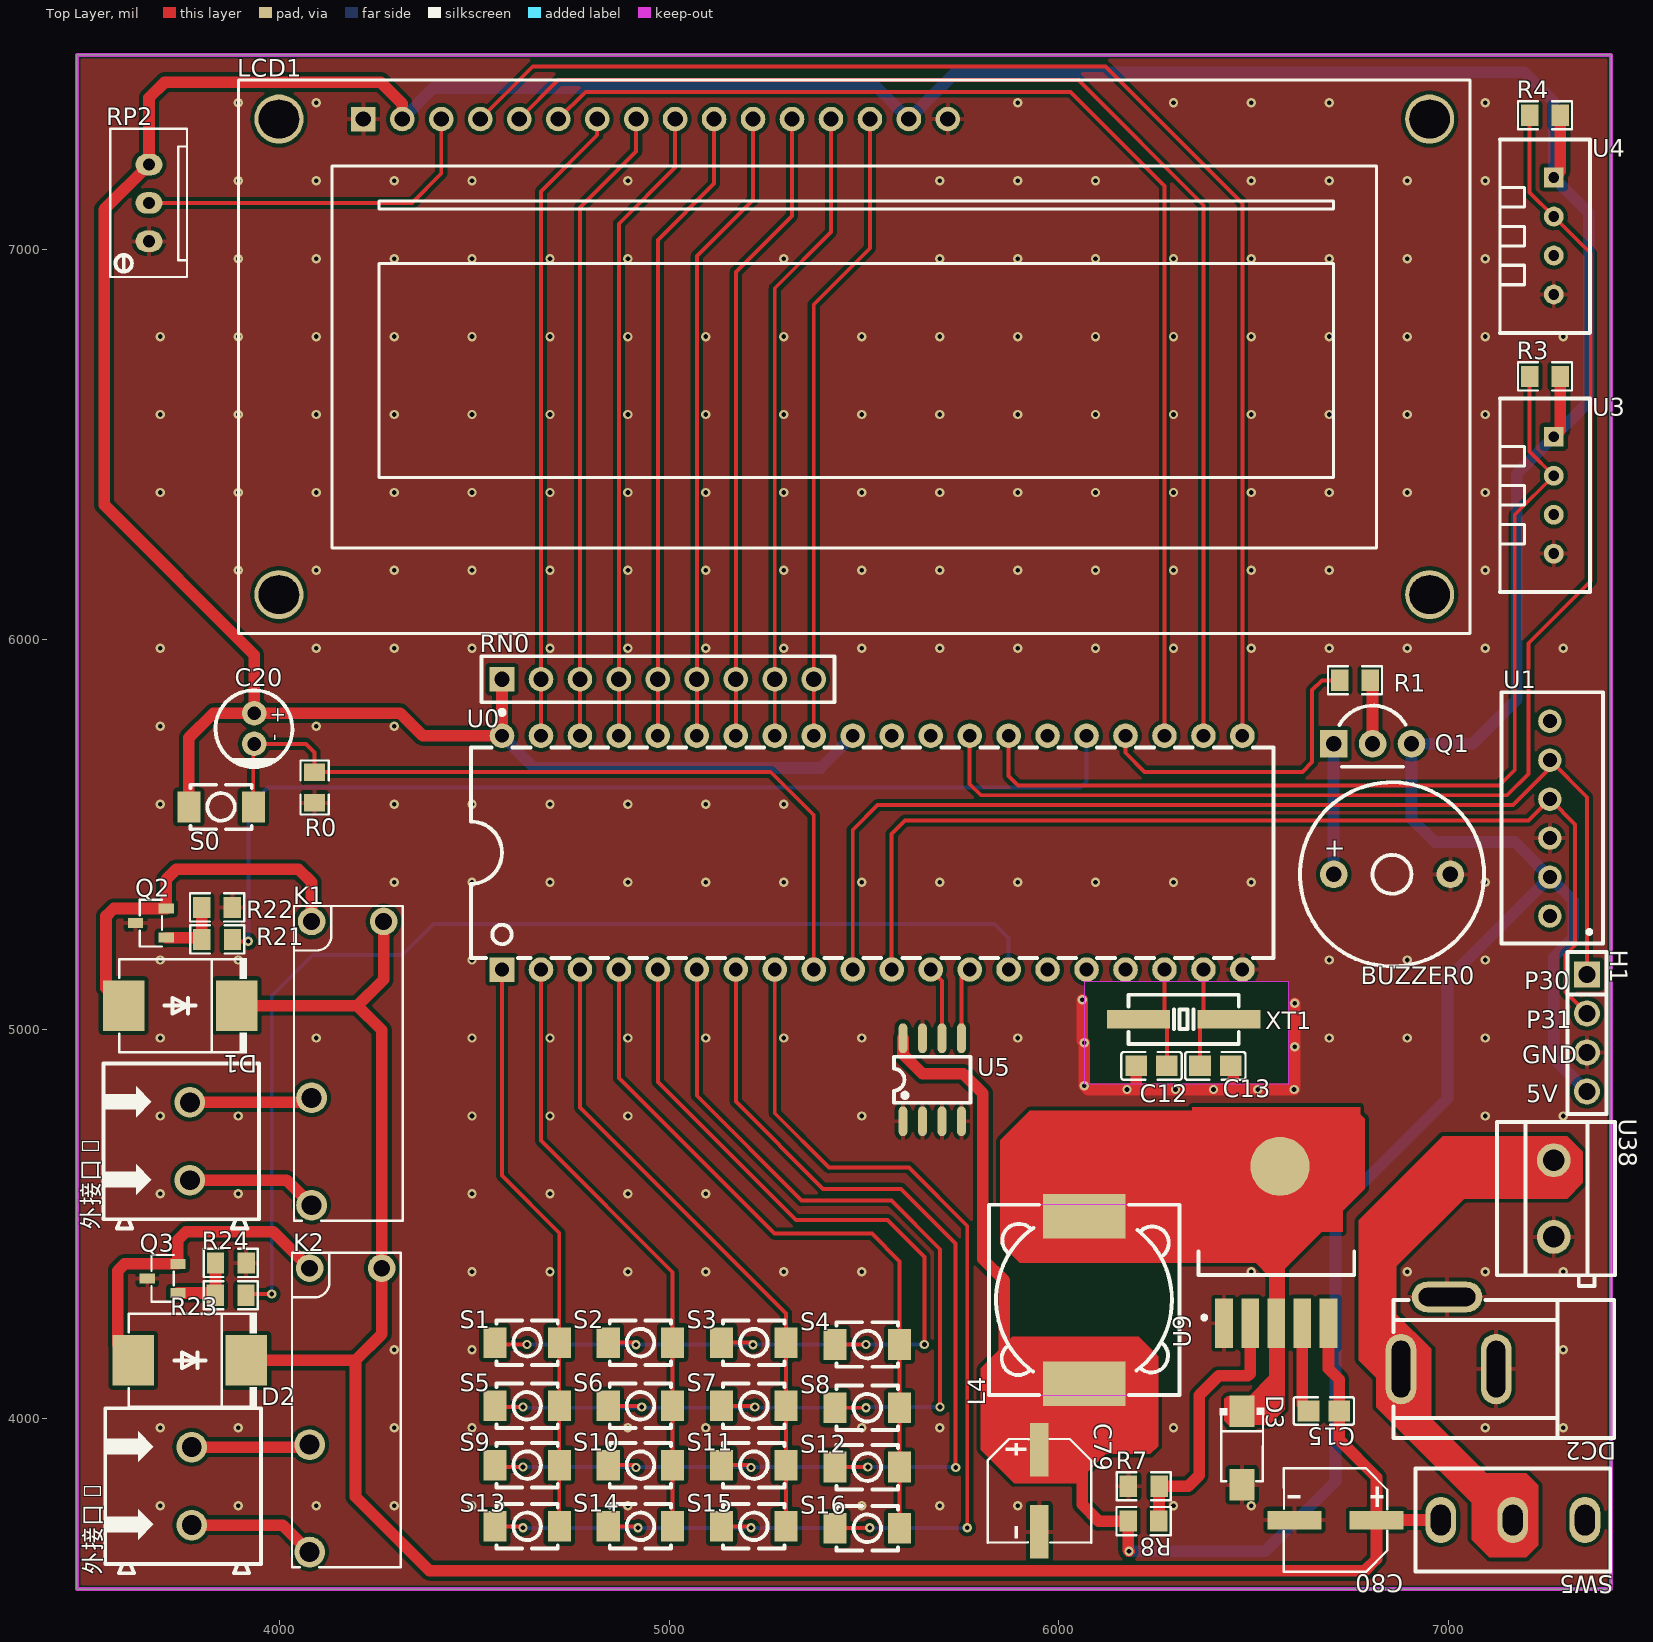
[diagram p0: Top Layer view]
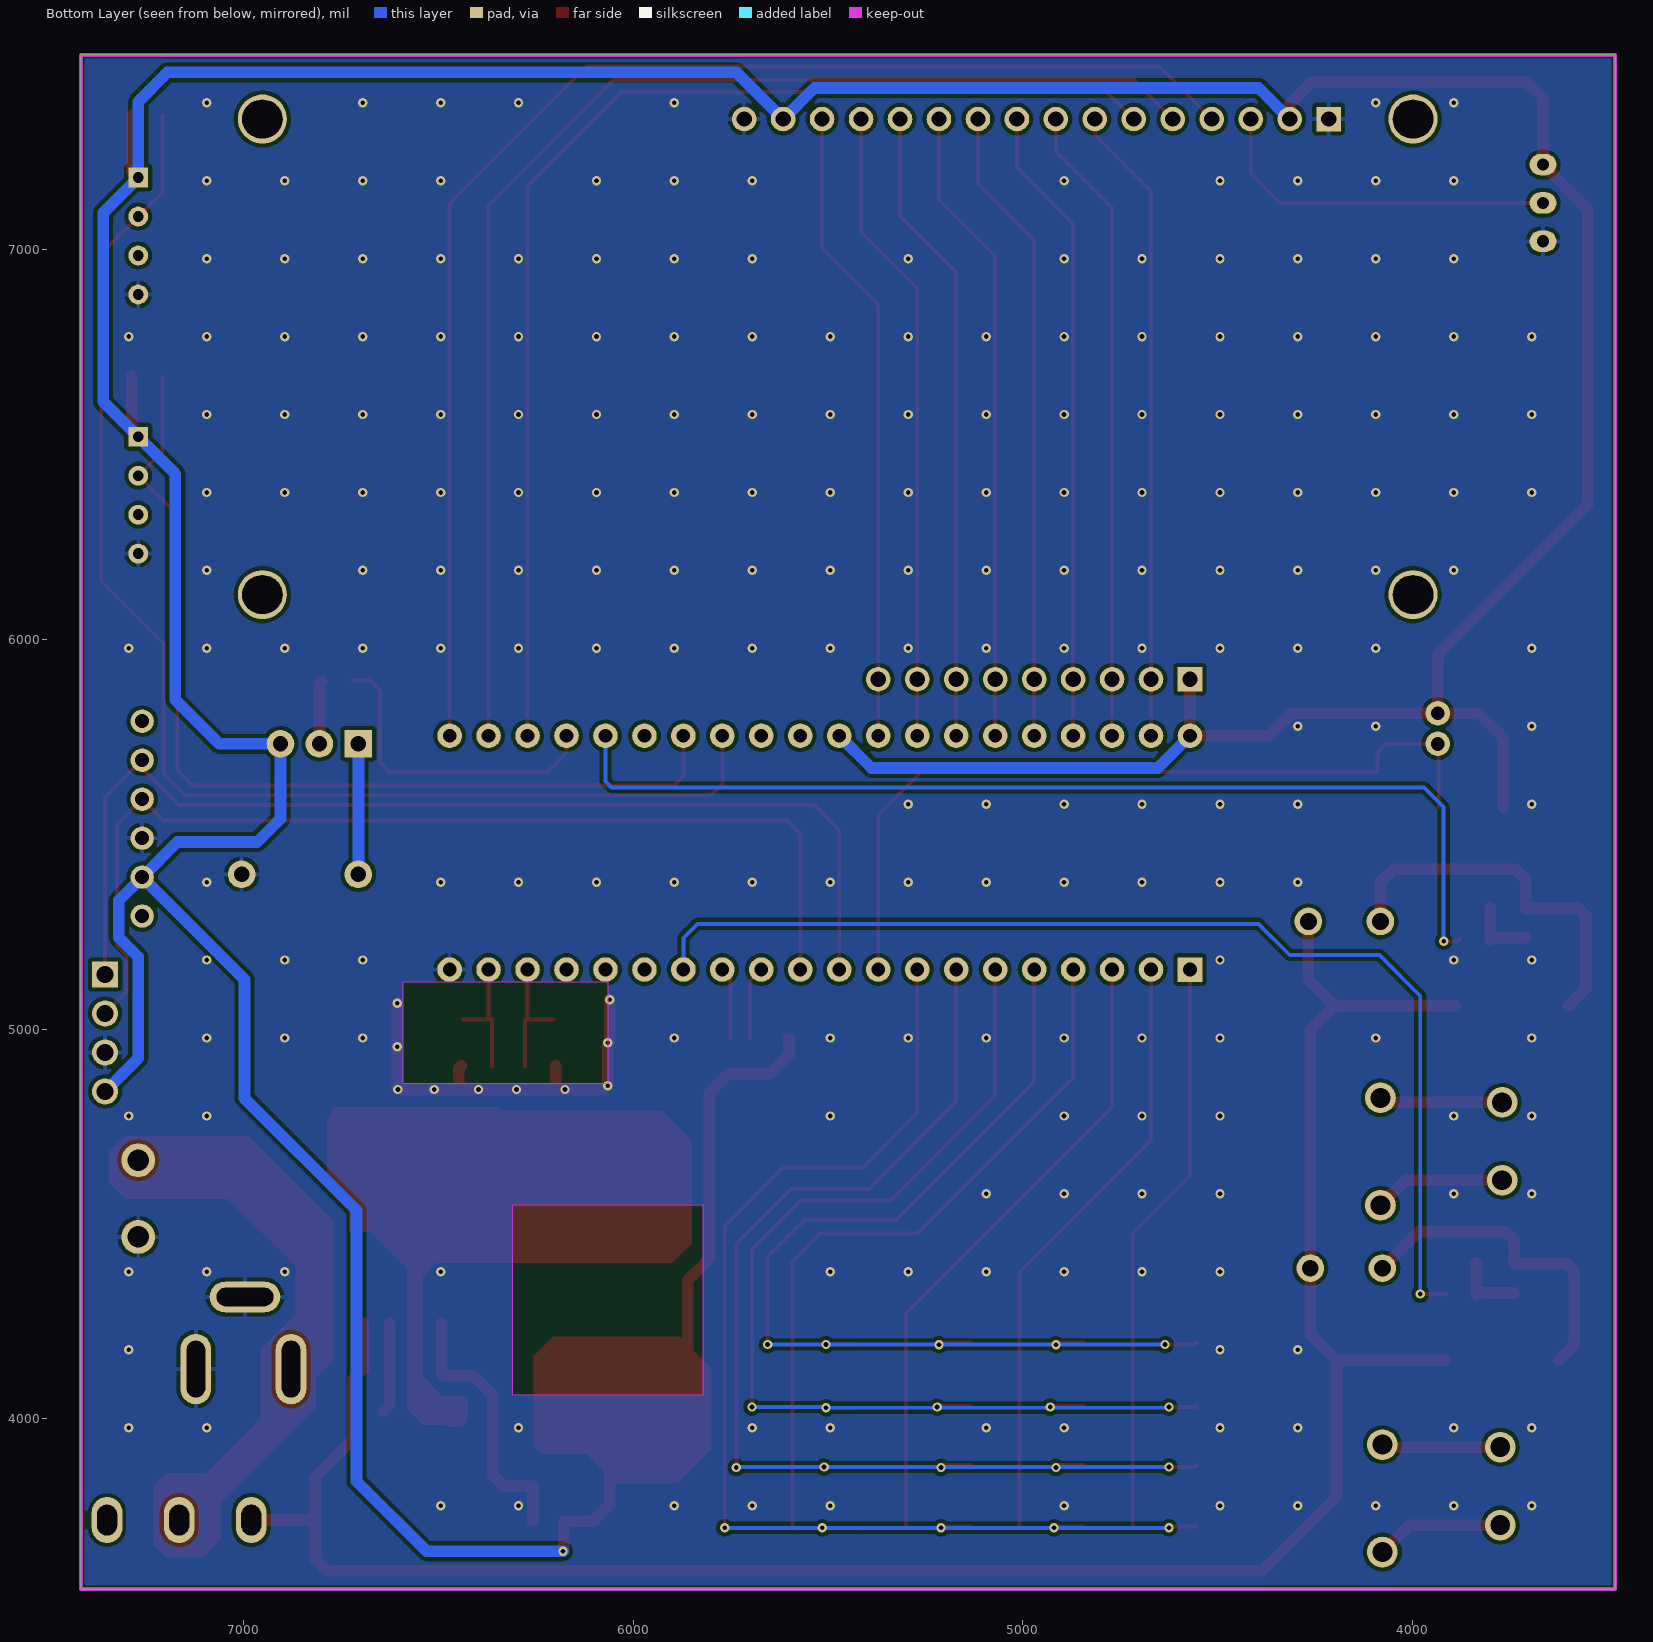
[diagram p1: Bottom Layer view, seen from below]
# Altium PCB MISC52141.pcbdoc
Units mil, origin at the board's own origin, x right, y up, seen from the top; angles counter-clockwise.
Board outline 3937.01 x 3937.01 mil, 2 copper layers (Top Layer, Bottom Layer), stack 62.206 mil thick; 59 components, 49 nets, 211 pads, 246 vias.

## Layer stack, top to bottom
Top Solder Mask Layer: solder mask 0.394, Dk 3.3
Top Layer: signal copper 1.379
Dielectric1: surface 59.449, FR4, Dk 4.5
Bottom Layer: signal copper 1.378
Bottom Solder Mask Layer: solder mask 0.394, Dk 3.3

## Board outline
3480,7500 3480,3562.99 7417.01,3562.99 7417.01,7500

## Design rules (kind name [scope] priority, off if disabled: settings)
BoardOutlineClearance copperThickness2oz_1 [All] p2 off: genericclearance=7.99 ignorepadtopadclearanceinfootprint=FALSE except(0: Arc-SplitContinuation Track-SplitContinuation SMDPad-SplitContinuation THPad-SplitContinuation Via-SplitContinuation Fill-SplitContinuation Region-SplitContinuation Poly-SplitContinuation Text-SplitContinuation Hole-SplitContinuation; 5.98: Arc-CutoutEdge SMDPad-CutoutEdge THPad-CutoutEdge Via-CutoutEdge Fill-CutoutEdge Region-CutoutEdge Text-CutoutEdge; 6.93: Hole-OutlineEdge Hole-CutoutEdge; 10: Poly-OutlineEdge Poly-CutoutEdge; 11.81: Arc-OutlineEdge Track-OutlineEdge SMDPad-OutlineEdge THPad-OutlineEdge Via-OutlineEdge Fill-OutlineEdge Region-OutlineEdge Text-OutlineEdge Track-CutoutEdge)
BoardOutlineClearance copperThickness1oz_1 [All] p4: genericclearance=4.02 ignorepadtopadclearanceinfootprint=FALSE except(0: Arc-SplitContinuation Track-SplitContinuation SMDPad-SplitContinuation THPad-SplitContinuation Via-SplitContinuation Fill-SplitContinuation Region-SplitContinuation Poly-SplitContinuation Text-SplitContinuation Hole-SplitContinuation; 6: SMDPad-CutoutEdge THPad-CutoutEdge Via-CutoutEdge Fill-CutoutEdge Region-CutoutEdge Text-CutoutEdge; 6.93: Hole-OutlineEdge Hole-CutoutEdge; 10: Poly-OutlineEdge Poly-CutoutEdge; 11.8: Arc-OutlineEdge Track-OutlineEdge SMDPad-OutlineEdge THPad-OutlineEdge Via-OutlineEdge Fill-OutlineEdge Region-OutlineEdge Text-OutlineEdge; 11.81: Arc-CutoutEdge Track-CutoutEdge)
Clearance copperThickness2oz [All] p1 off: gap=7.99 ignorepadtopadclearanceinfootprint=FALSE except(5.98: SMDPad-Track SMDPad-SMDPad THPad-Track SMDPad-THPad THPad-THPad Track-Via SMDPad-Via THPad-Via Via-Via Fill-Track Region-Track Fill-SMDPad Region-SMDPad Fill-THPad Region-THPad Fill-Via Region-Via Fill-Fill Fill-Region Region-Region Arc-Track Arc-SMDPad Arc-THPad Arc-Via Fill-Arc Region-Arc Arc-Arc Text-Track SMDPad-Text Text-THPad Text-Via Fill-Text Region-Text Arc-Text Text-Text; 6.93: Hole-Track Hole-SMDPad Hole-THPad Hole-Via Fill-Hole Region-Hole Hole-Arc Hole-Text; 10: Poly-Track Poly-SMDPad Poly-THPad Poly-Via Poly-Fill Poly-Region Poly-Poly Poly-Arc Poly-Text Poly-Hole)
Clearance copperThickness1oz [All] p3: gap=4.02 ignorepadtopadclearanceinfootprint=FALSE except(5.98: SMDPad-Track SMDPad-SMDPad THPad-Track SMDPad-THPad THPad-THPad Track-Via SMDPad-Via THPad-Via Via-Via Fill-Track Region-Track Fill-SMDPad Region-SMDPad Fill-THPad Region-THPad Fill-Via Region-Via Fill-Fill Fill-Region Region-Region; 6: Arc-Track Arc-SMDPad Arc-THPad Arc-Via Fill-Arc Region-Arc Arc-Arc Text-Track SMDPad-Text Text-THPad Text-Via Fill-Text Region-Text Arc-Text Text-Text; 6.93: Hole-Track Hole-SMDPad Hole-THPad Hole-Via Fill-Hole Region-Hole Hole-Arc Hole-Text; 10: Poly-Track Poly-SMDPad Poly-THPad Poly-Via Poly-Fill Poly-Region Poly-Poly Poly-Arc Poly-Text Poly-Hole)
DiffPairsRouting differentialPair [All] p1: maxlimit=6 minlimit=6 mostfreqgap=6 toplayer_minwidth=5 toplayer_prefwidth=10 toplayer_maxwidth=100 toplayer_mingap=6 toplayer_prefgap=6 toplayer_maxgap=6 bottomlayer_minwidth=5 bottomlayer_prefwidth=10 bottomlayer_maxwidth=100 bottomlayer_mingap=6 bottomlayer_prefgap=6 bottomlayer_maxgap=6 maxuncoupledlength=10
HoleToHoleClearance otherClearance [All] p1: gap=11.81 allowstackedmicrovias=TRUE
Length netLength [All] p1: minlimit=0 maxlimit=0
MatchedLengths netLengthTolerance [All] p1: tolerance=1000
PasteMaskExpansion pasteMaskExpansion [All] p1: expansion=0
PlaneConnect innerPlane [All] p1: planeconnectstyle=Relief reliefexpansion=20 reliefentries=4 reliefconductorwidth=10 reliefairgap=10
PolygonConnect copperRegion [(InNet('GND'))] p1: connectstyle=Relief reliefconductorwidth=10 reliefentries=4 polygonreliefangle="90 Angle" airgapwidth=10 via.connectstyle=Relief via.reliefconductorwidth=10 via.reliefentries=4 via.polygonreliefangle="90 Angle" via.airgapwidth=10
RoutingVias viaSize [All] p1: holewidth=12.01 width=24.02 viastyle="Through Hole" minholewidth=11.81 minwidth=19.68 maxholewidth=248.03 maxwidth=393.7
SolderMaskExpansion solderMaskExpansion [IsVia] p1: expansion=-1000 istentingtop=TRUE
SolderMaskExpansion solderMaskExpansion [All] p2: expansion=2 istentingtop=FALSE
Width copperThickness2oz_2 [All] p1 off: maxlimit=100 minlimit=8 preferedwidth=10
Width copperThickness1oz_2 [All] p2: maxlimit=100 minlimit=5 preferedwidth=10

## Components (designator, comment, footprint, x,y, rotation, side; value= is the part's Value field where it differs from the comment)
BUZZER0 "2.4kHz" BUZ-TH_BD12.0-P7.60-D0.6-FD 6855,5397.11 r0 top
C12 "30pf" C0805 6237.82,4905.52 r180 top
C13 "30pf" C0805 6401.58,4905.52 r0 top
C15 "100nF" C0805 6680,4020 r180 top
C20 "CAP-E" CAP-TH_BD5.0-P2.00-D0.5-FD-A 3935.01,5771.26 r270 top
C79 "100uF" CAP-SMD_BD6.3-L6.6-W6.6-LS7.4-FD 5950,3815 r270 top
C80 "100uF" CAP-SMD_BD6.3-L6.6-W6.6-LS7.4-FD 6710,3740 r180 top
D1 "" SMC_L6.9-W5.9-LS7.9-RD 3745,5060 r180 top
D2 "" SMC_L6.9-W5.9-LS7.9-RD 3770,4150 r180 top
D3 "SS510" SMA_L4.3-W2.6-LS5.0-RD 6470,3925 r270 top
DC2 "DC005" DC-IN-TH_DC005 7000,4220 r180 top
H1 "" HDR-TH_4P-P2.54-V-F 7355,4990 r270 top
K1 "" RELAY-TH_G5NB-1A-E-DCXX 4174.81,4912.09 r270 top
K2 "" RELAY-TH_G5NB-1A-E-DCXX 4169.81,4022.09 r270 top
L4 "47uH" IND-SMD_L12.3-W12.3 6065,4305 r90 top
LCD1 "LCD 1602" LCD1602 5475,6725 r0 top
Q1 "SS8550DTA" TO-92-3_L4.8-W3.7-P2.54-L 6805,5732.11 r0 top
Q2 "S8050(0.5A)" SOT-23-3_L2.9-W1.3-P1.90-LS2.4-BR 3669.81,5272.09 r0 top
Q3 "S8050(0.5A)" SOT-23-3_L2.9-W1.3-P1.90-LS2.4-BR 3700,4360 r0 top
R0 "10K" R0805 4090,5620 r90 top
R1 "5.1K" R0805 6760,5895 r0 top
R3 "10K" R0805 7247.35,6675 r0 top
R4 "10K" R0805 7247.35,7345 r0 top
R7 "3.3K" R0805 6217.85,3826.84 r0 top
R8 "10K" R0805 6217.38,3737.37 r180 top
R21 "4.7K" R0805 3840,5230 r0 top
R22 "4.7K" R0805 3839.81,5312.09 r180 top
R23 "4.7K" R0805 3874.81,4317.09 r0 top
R24 "4.7K" R0805 3875,4400 r180 top
RN0 "10kΩ" RES-ARRAY-TH_9P-P2.54-D1.0 4971,5897.74 r0 top
RP2 "10K" RES-ADJ-TH_3296W-1-203 3665,7119.99 r270 top
S0 "SW2" SW-SMD_L3.9-W2.9-LS5.0 3850,5570 r180 top
S1 "SW2" SW-SMD_L3.9-W2.9-LS5.0 4635.31,4195.44 r0 top
S2 "SW2" SW-SMD_L3.9-W2.9-LS5.0 4926.31,4195.44 r0 top
S3 "SW2" SW-SMD_L3.9-W2.9-LS5.0 5217.31,4195.44 r0 top
S4 "SW2" SW-SMD_L3.9-W2.9-LS5.0 5508.31,4190.44 r0 top
S5 "SW2" SW-SMD_L3.9-W2.9-LS5.0 4635.31,4033.23 r0 top
S6 "SW2" SW-SMD_L3.9-W2.9-LS5.0 4926.31,4033.23 r0 top
S7 "SW2" SW-SMD_L3.9-W2.9-LS5.0 5217.32,4033.23 r0 top
S8 "SW2" SW-SMD_L3.9-W2.9-LS5.0 5508.32,4028.23 r0 top
S9 "SW2" SW-SMD_L3.9-W2.9-LS5.0 4635.31,3881.03 r0 top
S10 "SW2" SW-SMD_L3.9-W2.9-LS5.0 4926.31,3881.03 r0 top
S11 "SW2" SW-SMD_L3.9-W2.9-LS5.0 5217.32,3881.03 r0 top
S12 "SW2" SW-SMD_L3.9-W2.9-LS5.0 5508.32,3876.03 r0 top
S13 "SW2" SW-SMD_L3.9-W2.9-LS5.0 4635.31,3723.82 r0 top
S14 "SW2" SW-SMD_L3.9-W2.9-LS5.0 4926.31,3723.82 r0 top
S15 "SW2" SW-SMD_L3.9-W2.9-LS5.0 5217.32,3723.82 r0 top
S16 "SW2" SW-SMD_L3.9-W2.9-LS5.0 5508.32,3718.82 r0 top
SW5 "SS-12D10L5" SW-TH_SS-12D10L5 7165,3740 r180 top
U0 "STC89C52RC-40I-PDIP40" DIP-40_L52.0-W13.7-P2.54-LS15.2-BL 5521,5452.74 r0 top
U1 "HM-10" HM-10.288 7260,5290 r180 top
U3 "DHT11" SENSOR-TH_DHT11 7270,6370 r270 top
U4 "DHT11" SENSOR-TH_DHT11 7270,7035 r270 top
U5 "M24C64-RMN6TP" SOIC-8_L5.0-W4.0-P1.27-LS6.0-BL 5675,4870 r0 top
U9 "XL4015E1" TO-263-5_L10.2-W8.9-P1.70-TL 6557.88,4442.34 r90 top
U38 "KF301-5.0-2P" CONN-TH_P5.00_KF301-5.0-2P 7270,4565 r270 top
XT1 "XT" HC-49S_L7.2-W3.2 6320,5025 r180 top
外接口1 "" CONN-TH_2P-P5.00_WJ500V-5.08-2P 3769.81,4712.09 r90 top
外接口2 "" CONN-TH_2P-P5.00_WJ500V-5.08-2P 3774.81,3827.09 r90 top

## Footprints (in the part's own frame and the unit in brackets; to place one, negate y for a bottom-side part, rotate by r counter-clockwise, add the part's x,y. Pads: shape width x height; smd on the part's side, far side on the other; paste and mask are expansions set on the pad)
BUZ-TH_BD12.0-P7.60-D0.6-FD [mm]
  round 1.8 hole 1: 1(-3.8,0) 2(3.8,0)
  silkscreen extent -6,-6 6,6
C0805 [mm]
  rect 1.41x1.35 smd paste-100 mask+0.051: 1(-1,0) 2(1,0)
  silkscreen extent -1.96,-0.9 1.96,0.9
CAP-SMD_BD6.3-L6.6-W6.6-LS7.4-FD [mm]
  rect 3.5x1.2 smd: 1(-2.67,0) 2(2.67,0)
  silkscreen extent -3.38,-3.38 3.38,3.38
CAP-TH_BD5.0-P2.00-D0.5-FD-A [mm]
  round 1.6 hole 0.9 paste+0 mask+0.05: 1(-1,0) 2(1,0)
  silkscreen extent -2.49,-2.52 2.6,2.49
CONN-TH_2P-P5.00_WJ500V-5.08-2P [mm]
  round 2 hole 1.3: 1(-2.54,0) 2(2.54,0)
  silkscreen extent -5.68,-4.52 5.08,5.64
CONN-TH_P5.00_KF301-5.0-2P [mm]
  round 2.2 hole 1.4: 1(-2.5,0) 2(2.5,0)
  silkscreen extent -5,-3.7 5.71,4
DC-IN-TH_DC005 [mm]
  oval 2x4.6 hole 1.2 slot 3.7 at 90 deg: 1(3.1,2.35) 2(-3.1,2.35)
  oval 4.6x2 hole 1.2 slot 3.7 at 0 deg: 3(0.1,-2.35)
  silkscreen extent -10.8,-2.15 3.6,6.85
DIP-40_L52.0-W13.7-P2.54-LS15.2-BL [mil]
  rect 63x63 hole 35: 1(-950,-300)
  round 63 hole 35: 2(-850,-300) 3(-750,-300) 4(-650,-300) 5(-550,-300) 6(-450,-300) 7(-350,-300) 8(-250,-300) 9(-150,-300) 10(-50,-300) 11(50,-300) 12(150,-300) 13(250,-300) 14(350,-300) 15(450,-300) 16(550,-300) 17(650,-300) 18(750,-300) 19(850,-300) 20(950,-300) 21(950,300) 22(850,300) 23(750,300) 24(650,300) 25(550,300) 26(450,300) 27(350,300) 28(250,300) 29(150,300) 30(50,300) 31(-50,300) 32(-150,300) 33(-250,300) 34(-350,300) 35(-450,300) 36(-550,300) 37(-650,300) 38(-750,300) 39(-850,300) 40(-950,300)
  silkscreen extent -1030,-270 1030,270
HC-49S_L7.2-W3.2 [mm]
  rect 4.1x1.2 smd: 1(-2.95,0) 2(2.95,0)
  silkscreen extent -3.6,-1.6 3.6,1.6
HDR-TH_4P-P2.54-V-F [mm]
  rect 1.7x1.7 hole 1.1: 1(-3.81,0)
  round 1.7 hole 1.1: 2(-1.27,0) 3(1.27,0) 4(3.81,0)
  silkscreen extent -5.29,-1.27 5.29,1.27
HM-10.288 [mil]
  round 60 hole 36: 1(0,0) 2(0,-100) 3(0,-200) 4(0,-300) 5(0,-400) 6(0,-500)
  silkscreen extent -136,-574 124,71
IND-SMD_L12.3-W12.3 [mm]
  rect 2.9x5.4 smd: 1(-5.45,0) 2(5.45,0)
  silkscreen extent -6.2,-6.2 6.2,6.2
LCD1602 [mm]
  round 3.2 hole 2.5 slot 2.625 at 0 deg: 0(-37.5,-15.5) 0(-37.5,15.5) 0(37.5,-15.5) 0(37.5,15.5)
  rect 1.6x1.6 hole 1: 1(-32,15.5)
  round 1.6 hole 1: 2(-29.46,15.5) 3(-26.92,15.5) 4(-24.38,15.5) 5(-21.84,15.5) 6(-19.3,15.5) 7(-16.76,15.5) 8(-14.22,15.5) 9(-11.68,15.5) 10(-9.14,15.5) 11(-6.6,15.5) 12(-4.06,15.5) 13(-1.52,15.5) 14(1.02,15.5) 15(3.56,15.5) 16(6.1,15.5)
  silkscreen extent -40.13,-18.03 40.13,18.03
R0805 [mm]
  rect 1.133x1.377 smd paste-100 mask+0.051: 1(-1,0) 2(1,0)
  silkscreen extent -1.76,-0.92 1.76,0.92
RELAY-TH_G5NB-1A-E-DCXX [mm]
  round 1.8 hole 1.1: 1(-9.25,-2.35) 4(-9.25,2.35)
  round 2 hole 1.3: 2(2.25,-2.35) 3(9.25,-2.35)
  silkscreen extent -10.25,-3.5 10.25,3.6
RES-ADJ-TH_3296W-1-203 [mm]
  oval 1.4x1.75 hole 0.8: 1(-2.5,0) 2(0,0) 3(2.5,0)
  silkscreen extent -4.83,-2.53 4.83,2.48
RES-ARRAY-TH_9P-P2.54-D1.0 [mm]
  rect 1.6x1.6 hole 1: 1(-10.16,0)
  round 1.6 hole 1: 2(-7.62,0) 3(-5.08,0) 4(-2.54,0) 5(0,0) 6(2.54,0) 7(5.08,0) 8(7.62,0) 9(10.16,0)
  silkscreen extent -11.5,-2.31 11.5,1.5
SENSOR-TH_DHT11 [mil]
  rect 51x51 hole 28: 1(-150,0)
  round 51 hole 28: 2(-50,0) 3(50,0) 4(150,0)
  silkscreen extent -248,-138 248,93
SMA_L4.3-W2.6-LS5.0-RD [mm]
  rect 2.046x1.62 smd: 1(-2.404,-0.009) 2(2.404,0.009)
  silkscreen extent -2.61,-1.44 2.16,1.44
SMC_L6.9-W5.9-LS7.9-RD [mm]
  rect 2.7x3.3 smd: 1(-3.686,0) 2(3.686,0)
  silkscreen extent -4.36,-3.1 3.98,3.1
SOIC-8_L5.0-W4.0-P1.27-LS6.0-BL [mil]
  oval 22.38x76.78 smd: 1(-75,-106.5) 2(-25,-106.5) 3(25,-106.5) 4(75,-106.5) 5(75,106.5) 6(25,106.5) 7(-25,106.5) 8(-75,106.5)
  silkscreen extent -98,-59 98,59
SOT-23-3_L2.9-W1.3-P1.90-LS2.4-BR [mm]
  rect 1x0.65 smd: 1(1,-0.95) 2(1,0.95) 3(-1,0)
  silkscreen extent -0.73,-1.53 0.73,1.53
SW-SMD_L3.9-W2.9-LS5.0 [mm]
  rect 1.5x2 smd: 1(-2.1,0) 2(2.1,0)
  silkscreen extent -2,-1.45 2,1.45
SW-TH_SS-12D10L5 [mm]
  oval 2x3 hole 1.3 slot 2 at 90 deg: 1(-4.7,0) 2(0,0) 3(4.7,0)
  silkscreen extent -6.35,-3.35 6.35,3.35
TO-92-3_L4.8-W3.7-P2.54-L [mm]
  rect 1.8x1.8 hole 1: 1(-2.54,0)
  round 1.8 hole 1: 2(0,0) 3(2.54,0)
  silkscreen extent -2.17,-1.5 2.14,2.48
TO-263-5_L10.2-W8.9-P1.70-TL [mm]
  rect 3.2x1.15 smd: 1(-5.008,3.404) 2(-5.008,1.702) 3(-5.008,0) 4(-5.008,-1.702) 5(-5.008,-3.404)
  round 3.852 smd: 6(5.219,-0.241)
  Top Layer region: 0.944,3.683 7.548,3.683 7.548,5.461 9.072,5.461 9.072,-5.461 7.548,-5.461 7.548,-4.317 0.944,-4.317
  silkscreen extent -4.77,-5.08 -0.33,5.08

## Via types
v1: diameter 24.02, hole 12, Top Layer to Bottom Layer, 246 vias

## Nets (pads, with @x,y where several pads share a name; then routed paths per layer and width w, separated by ;. In a path a pad name is that pad's centre, name@x,y a point inside that pad or via, vN(x,y) a via of type N, cw(c..) or ccw(c..) an arc to the next point about the centre after c; other vN are vias at no path point)
12V: C15.1 C80.1 D1.1 D2.1 K1.4 K2.4 SW5.3 U9.5 | length 5679.8
  Top Layer w30: D1.1 4200,5060 ; D2.1 4195,4150 ; K1.4 4267.33,5127.33 4200,5060 ; U9.5 6691.88,4128.12 6719.37,4100.63 C15.1 6719.37,3945.63 6815.11,3849.89 C80.1 ; SW5.3 C80.1 ; 4195,4150 4262.33,4217.33 K2.4 4262.33,4997.67 4200,5060 ; 4195,4150 4195,3800 4385,3610 6785,3610 6815.11,3640.11 C80.1
$1N45: C20.2 R0.2 S0.1 U0.9 | length 2100.5
  Top Layer w10: S0.1 3932.68,5729.57 C20.2 4068.11,5731.89 4090,5710 R0.2 5260.63,5659.37 5371,5549 U0.9
$1N63: LCD1.3 RP2.2 | length 921.4
  Top Layer w10: RP2.2 4339.99,7119.99 4415.16,7195.16 LCD1.3
$1N105: Q1.2 R1.2 | length 162.3
  Top Layer w30: R1.2@6799.37,5892.11 6805,5886.48 Q1.2
$1N108: BUZZER0.1 Q1.1 | length 335.2
  Bottom Layer w30: Q1.1 6705,5397.51 BUZZER0.1
$1N929: K1.2 外接口1.2 | length 317.2
  Top Layer w30: 外接口1.2 4070.87,4812.09 K1.2
$1N930: K1.3 外接口1.1 | length 339.1
  Top Layer w30: 外接口1.1 4018.11,4612.09 K1.3
$1N931: D1.2 K1.1 Q2.2 | length 983.4
  Top Layer w30: D1.2 3555,5104.87 3555,5290 3574.49,5309.49 Q2.2 3709.18,5384.18 3735,5410 4048.79,5410 4082.29,5376.5 K1.1
$1N934: Q2.1 R21.1 R22.2 | length 175.3
  Top Layer w30: Q2.1 3795.94,5234.69 R21.1@3800.44,5230.19 ; R22.2 R21.1@3800.44,5230.19 ; R21.1 R21.1@3800.44,5230.19
$1N936: K2.2 外接口2.2 | length 305.1
  Top Layer w30: 外接口2.2 4070.87,3927.09 K2.2
$1N937: K2.3 外接口2.1 | length 331.1
  Top Layer w30: 外接口2.1 4008.11,3727.09 K2.3
$1N938: D2.2 K2.1 Q3.2 | length 855.8
  Top Layer w30: D2.2 3585,4189.87 3585,4380 3602.4,4397.4 Q3.2 3738.79,4397.98 3738.79,4458.79 3760,4480 3983.55,4480 K2.1
$1N941: Q3.1 R23.1 R24.2 | length 181.3
  Top Layer w30: Q3.1 3829.92,4322.6 R23.1 3835.63,4317.28 R24.2
$1N950: D3.1 L4.2 U9.3 U9.6 | length 1244.7
  Top Layer w30: L4.2 6450.45,4519.57 U9.6@6557.88,4627 ; D3.1 6544.65,4019.64 6560,4035 6560,4243.07 U9.3 U9.6@6557.88,4627 ; U9.6@6570.38,4639.5 U9.6@6557.88,4627
$1N952: C15.2 U9.4 | length 231.7
  Top Layer w30: U9.4 6624.88,4035.75 C15.2
$1N964: DC2.1 SW5.2 U38.1
+5V: C20.1 C79.1 H1.4 L4.1 LCD1.2 LCD1.15 Q1.3 R3.2 R4.2 R8.2 RN0.1 RP2.1 S0.2 U0.31 U0.40 U1.2 U3.1 U4.1 U5.8 | length 15136.3
  Top Layer w30: S0.2 3767.32,5747.32 3830.63,5810.63 C20.1 ; LCD1.2 4315.16,7374.84 4260,7430 3705,7430 3665,7390 RP2.1 3550,7103.41 3550,6345 3935,5960 C20.1 ; RN0.1 U0.40 4367.26,5752.74 4309.37,5810.63 C20.1 ; U5.8 5600,4935 5650,4885 5755,4885 5805,4835 5805,4410 5860,4355 5860,4120 ; C79.1 6004.89,3920.11 6060,3865 6060,3780 6102.63,3737.37 R8.2 6178.01,3661.99 v1(6180,3660) ; U3.1 7286.72,6536.72 R3.2 ; U4.1 7286.72,7201.72 R4.2
  Bottom Layer w30: LCD1.2 4394.92,7415 5535.4,7415 LCD1.15 5734.92,7455 7195,7455 7270,7380 U4.1 7360,7095 7360,6610 U3.1 7175,6425 7175,5845 7062.11,5732.11 Q1.3 6905,5540 6965,5480 7170,5480 U1.2 ; U0.40 4653.74,5670 5388.26,5670 U0.31 ; v1(6180,3660) 6530,3660 6710,3840 6710,4535 6997.5,4822.5 6997.5,5127.5 U1.2 ; H1.4 7270,4925 7270,5185 7320,5235 7320,5330 U1.2
FB: R7.2 R8.1 U9.2 | length 692.4
  Top Layer w30: R8.1 6256.75,3826.37 R7.2 6331.84,3826.84 6360,3855 6360,4060 6410,4110 6485,4110 6490.88,4115.88 U9.2
GND: BUZZER0.2 C12.2 C13.2 C79.2 C80.2 D3.2 DC2.2 DC2.3 H1.3 LCD1.1 LCD1.16 Q2.3 Q3.3 R0.1 R7.1 R22.1 R24.1 RP2.3 U0.20 U1.3 U3.4 U4.4 U5.1 U5.2 U5.3 U5.4 U5.7 U9.1 U38.2 | length 1110.9
  Top Layer w30: v1(6060,5075) 6060,4970 v1(6065,4965) v1(6065,4854.78) 6074.78,4845 v1(6175,4845) 6196.99,4845 ; C12.2 6198.45,4846.46 6196.99,4845 ; C13.2 6447.41,4899.06 6447.41,4845 ; v1(6605,5066.04) v1(6605,4955) 6605,4846.4 v1(6603.6,4845) v1(6510.71,4845) 6447.41,4845 ; 6196.99,4845 v1(6299.45,4845) v1(6396.88,4845) 6447.41,4845
  other v1: 3694.1,3777.09 3894.1,3777.09 4094.1,3777.09 4294.1,3777.09 4494.1,3777.09 4894.1,3777.09 5494.1,3777.09 5694.1,3777.09 5894.1,3777.09 6294.1,3777.09 6494.1,3777.09 3694.1,3977.09 3894.1,3977.09 4294.1,3977.09 4494.1,3977.09 4894.1,3977.09 5094.1,3977.09 5494.1,3977.09 5694.1,3977.09 6294.1,3977.09 7094.1,3977.09 7294.1,3977.09 4294.1,4177.09 4494.1,4177.09 7294.1,4177.09 4494.1,4377.09 4694.1,4377.09 4894.1,4377.09 5094.1,4377.09 5294.1,4377.09 5494.1,4377.09 6494.1,4377.09 6894.1,4377.09 7094.1,4377.09 7294.1,4377.09 3694.1,4577.09 3894.1,4577.09 4494.1,4577.09 4694.1,4577.09 4894.1,4577.09 5094.1,4577.09 3694.1,4777.09 3894.1,4777.09 4494.1,4777.09 4694.1,4777.09 4894.1,4777.09 5494.1,4777.09 7094.1,4777.09 7294.1,4777.09 3694.1,4977.09 4094.1,4977.09 4494.1,4977.09 4694.1,4977.09 4894.1,4977.09 5094.1,4977.09 5294.1,4977.09 5494.1,4977.09 5894.1,4977.09 6694.1,4977.09 6894.1,4977.09 7094.1,4977.09 3694.1,5177.09 3894.1,5177.09 4494.1,5177.09 6694.1,5177.09 6894.1,5177.09 7094.1,5177.09 4294.1,5377.09 4494.1,5377.09 4694.1,5377.09 4894.1,5377.09 5094.1,5377.09 5294.1,5377.09 5494.1,5377.09 5694.1,5377.09 5894.1,5377.09 6094.1,5377.09 6294.1,5377.09 6494.1,5377.09 7094.1,5377.09 3694.1,5577.09 4294.1,5577.09 4494.1,5577.09 4694.1,5577.09 4894.1,5577.09 5094.1,5577.09 5294.1,5577.09 3694.1,5777.09 4094.1,5777.09 4294.1,5777.09 3694.1,5977.09 4094.1,5977.09 4294.1,5977.09 4494.1,5977.09 4694.1,5977.09 4894.1,5977.09 5094.1,5977.09 5294.1,5977.09 5494.1,5977.09 5694.1,5977.09 5894.1,5977.09 6094.1,5977.09 6294.1,5977.09 6494.1,5977.09 6694.1,5977.09 6894.1,5977.09 7094.1,5977.09 7294.1,5977.09 3894.1,6177.09 4094.1,6177.09 4294.1,6177.09 4494.1,6177.09 4694.1,6177.09 4894.1,6177.09 5094.1,6177.09 5294.1,6177.09 5494.1,6177.09 5694.1,6177.09 5894.1,6177.09 6094.1,6177.09 6294.1,6177.09 6494.1,6177.09 6694.1,6177.09 7094.1,6177.09 3694.1,6377.09 3894.1,6377.09 4094.1,6377.09 4294.1,6377.09 4494.1,6377.09 4694.1,6377.09 4894.1,6377.09 5094.1,6377.09 5294.1,6377.09 5494.1,6377.09 5694.1,6377.09 5894.1,6377.09 6094.1,6377.09 6294.1,6377.09 6494.1,6377.09 6694.1,6377.09 6894.1,6377.09 7094.1,6377.09 3694.1,6577.09 3894.1,6577.09 4094.1,6577.09 4294.1,6577.09 4494.1,6577.09 4694.1,6577.09 4894.1,6577.09 5094.1,6577.09 5294.1,6577.09 5494.1,6577.09 5694.1,6577.09 5894.1,6577.09 6094.1,6577.09 6294.1,6577.09 6494.1,6577.09 6694.1,6577.09 6894.1,6577.09 7094.1,6577.09 3694.1,6777.09 3894.1,6777.09 4094.1,6777.09 4294.1,6777.09 4494.1,6777.09 4694.1,6777.09 4894.1,6777.09 5094.1,6777.09 5294.1,6777.09 5494.1,6777.09 5694.1,6777.09 5894.1,6777.09 6094.1,6777.09 6294.1,6777.09 6494.1,6777.09 6694.1,6777.09 6894.1,6777.09 7094.1,6777.09 7294.1,6777.09 3894.1,6977.09 4094.1,6977.09 4294.1,6977.09 4494.1,6977.09 4694.1,6977.09 4894.1,6977.09 5294.1,6977.09 5694.1,6977.09 5894.1,6977.09 6094.1,6977.09 6294.1,6977.09 6494.1,6977.09 6694.1,6977.09 6894.1,6977.09 7094.1,6977.09 3894.1,7177.09 4094.1,7177.09 4294.1,7177.09 4494.1,7177.09 4894.1,7177.09 5694.1,7177.09 5894.1,7177.09 6094.1,7177.09 6494.1,7177.09 6694.1,7177.09 6894.1,7177.09 7094.1,7177.09 3894.1,7377.09 4094.1,7377.09 5894.1,7377.09 6294.1,7377.09 6494.1,7377.09 6694.1,7377.09 7094.1,7377.09
P00: LCD1.7 RN0.2 U0.39 | length 1642.2
  Top Layer w10: U0.39 RN0.2 4671,7149.58 4815.16,7293.74 LCD1.7
P01: LCD1.8 RN0.3 U0.38 | length 1642.2
  Top Layer w10: U0.38 RN0.3 4771,7108.16 4915.16,7252.32 LCD1.8
P02: LCD1.9 RN0.4 U0.37 | length 1642.2
  Top Layer w10: U0.37 RN0.4 4871,7066.74 5015.16,7210.9 LCD1.9
P03: LCD1.10 RN0.5 U0.36 | length 1642.2
  Top Layer w10: U0.36 RN0.5 4971,7025.32 5115.16,7169.48 LCD1.10
P04: LCD1.11 RN0.6 U0.35 | length 1642.2
  Top Layer w10: U0.35 RN0.6 5071,6983.9 5215.16,7128.06 LCD1.11
P05: LCD1.12 RN0.7 U0.34 | length 1642.2
  Top Layer w10: U0.34 RN0.7 5171,6942.48 5315.16,7086.64 LCD1.12
P06: LCD1.13 RN0.8 U0.33 | length 1642.2
  Top Layer w10: U0.33 RN0.8 5271,6901.05 5415.16,7045.22 LCD1.13
P07: LCD1.14 RN0.9 U0.32 | length 1642.2
  Top Layer w10: U0.32 RN0.9 5371,6859.63 5515.16,7003.79 LCD1.14
P10: S1.2 S5.2 S9.2 S13.2 U0.1 | length 1489.8
  Top Layer w10: U0.1 4571,4624 4717.99,4477.01 S1.2 S5.2 S9.2 S13.2
P11: S2.2 S6.2 S10.2 S14.2 U0.2 | length 1568.9
  Top Layer w10: U0.2 4671,4714 5008.99,4376.01 S2.2 S6.2 S10.2 S14.2
P12: S3.2 S7.2 S11.2 S15.2 U0.3 | length 1648
  Top Layer w10: U0.3 4771,4799 5299.99,4270.01 S3.2 S7.2 S11.2 S15.2
P13: S4.2 S8.2 S12.2 S16.2 U0.4 | length 1878.6
  Top Layer w10: U0.4 4871,4874 5270,4475 5520,4475 5590.99,4404.01 S4.2 S8.2 S12.2 S16.2
P14: S1.1 S2.1 S3.1 S4.1 U0.5 | length 2723.3
  Top Layer w10: S1.1 4557.63,4190.44 v1(4635,4190.44) ; S2.1 4909.56,4195.44 v1(4915,4190) ; U0.5 4971,4864 5325,4510 5560,4510 5655,4415 v1(5655,4190.44) ; S3.1 5209.56,4195.44 v1(5215,4190) ; S4.1 v1(5505,4190.44)
  Bottom Layer w10: v1(4635,4190.44) v1(5505,4190.44) v1(5655,4190.44)
P15: S5.1 S6.1 S7.1 S8.1 U0.6 | length 2914.9
  Top Layer w10: S5.1 4555.86,4030 v1(4625,4030) ; S6.1 4926.77,4033.23 v1(4930,4030) ; U0.6 5071,4829 5340,4560 5570,4560 5695,4435 v1(5695,4030) ; S7.1 5216.77,4033.23 v1(5220,4030) ; S8.1 v1(5505,4028.23)
  Bottom Layer w10: v1(4625,4030) 4626.77,4028.23 v1(5505,4028.23) 5506.77,4030 v1(5695,4030)
P16: S9.1 S10.1 S11.1 S12.1 U0.7 | length 3049.5
  Top Layer w10: S9.1 4557.63,3876.03 v1(4625,3876.03) ; S10.1 4908.97,3881.03 v1(4915,3875) ; S11.1 5203.97,3881.03 v1(5210,3875) ; U0.7 5171,4814 5395,4590 5595,4590 5735,4450 v1(5735,3875) ; S12.1 v1(5510,3876.03)
  Bottom Layer w10: v1(4625,3876.03) v1(5510,3876.03) 5733.97,3876.03 v1(5735,3875)
P17: S13.1 S14.1 S15.1 S16.1 U0.8 | length 3216.2
  Top Layer w10: S13.1 4621.18,3723.82 v1(4625,3720) ; S14.1 4916.18,3723.82 v1(4920,3720) ; S15.1 5206.18,3723.82 v1(5210,3720) ; U0.8 5271,4784 5410,4645 5615,4645 5765,4495 v1(5765,3720) ; S16.1 5426.82,3720 v1(5515,3720)
  Bottom Layer w10: v1(4625,3720) v1(4920,3720) v1(5210,3720) v1(5515,3720) v1(5765,3720)
P20: LCD1.4 U0.21 | length 3523.3
  Top Layer w10: LCD1.4 4649.92,7470 6120,7470 6471,7119 U0.21
P21: LCD1.5 U0.22 | length 3291.4
  Top Layer w10: LCD1.5 4714.92,7435 6050,7435 6371,7114 U0.22
P22: LCD1.6 U0.23 | length 3095.8
  Top Layer w10: LCD1.6 4784.92,7405 6030,7405 6271,7164 U0.23
P23: R1.1 U0.24 | length 819.4
  Top Layer w10: U0.24 6171,5709 6220,5660 6625,5660 6650,5685 6650,5870 6675,5895 R1.1
P24: R21.2 U0.25 | length 2682.8
  Top Layer w10: R21.2 3884.37,5225 v1(3920,5225)
  Bottom Layer w10: v1(3920,5225) 3920,5570 3970,5620 6055,5620 6071,5636 U0.25
P26: R3.1 U0.27 U3.2 | length 2506.4
  Top Layer w10: U0.27 5871,5649 5895,5625 7130,5625 7170,5665 7170,6320 U3.2 7207.98,6482.02 R3.1
P27: R4.1 U0.28 U4.2 | length 3413.8
  Top Layer w10: U0.28 5771,5629 5800,5600 7150,5600 7205,5655 7205,5990 7365,6150 7365,6990 U4.2 7207.98,7147.02 R4.1
P30: H1.1 U0.10 U1.5 | length 2822.5
  Top Layer w10: U0.10 5471,5511 5535,5575 7165,5575 7260,5670 U1.5 7355,5595 H1.1
P31: H1.2 U0.11 U1.4 | length 2684.2
  Top Layer w10: U0.11 5571,5501 5605,5535 7205,5535 U1.4 7325,5525 7325,5215 7300,5190 7300,5095 H1.2
P32: U0.12 U5.6 | length 188.3
  Top Layer w10: U0.12 5700,5123.74 U5.6
P33: U0.13 U5.5 | length 184.9
  Top Layer w10: U5.5 5750,5131.74 U0.13
P34: R23.2 U0.14 | length 2895.8
  Top Layer w10: R23.2 3917.09,4320 v1(3980,4320)
  Bottom Layer w10: v1(3980,4320) 3980,5085 4085,5190 4315,5190 4395,5270 5835,5270 5871,5234 U0.14
XTAL1: C12.1 U0.18 XT1.2 | length 320.6
  Top Layer w10: XT1.2 XT1.2@6271,5025 ; U0.18 XT1.2@6271,5025 ; C12.1 6277.19,5025 XT1.2@6271,5025
XTAL2: C13.1 U0.19 XT1.1 | length 321.1
  Top Layer w10: C13.1 6362.21,5025 XT1.1@6371,5025 ; U0.19 XT1.1@6371,5025 ; XT1.1 XT1.1@6371,5025
pads on no net: LCD1.0 SW5.1 U0.15 U0.16 U0.17 U0.26 U0.29 U0.30 U1.1 U1.6 U3.3 U4.3

## Polygon pours and split planes (outlines as drawn)
GND on Top Layer (solid, remove dead copper, pour order 0): 3000,7700 3000,3000 7675,3000 7675,7700
GND on Bottom Layer (solid, remove dead copper, pour order 2): 3275,7780 3275,3225 7840,3225 7840,7780

## Keep-outs
Board Outline Layer:
  region: 5820.91,4549.09 5820.91,4060.9 6309.09,4060.9 6309.09,4549.09
  region: 6065,5121.37 6065,4860 6590,4860 6590,5121.37
  lines w10: 3480,3562.99 3480,7500 7417.01,7500 7417.01,3562.99 3480,3562.99

## Other copper
Top Layer:
  region net $1N964: 7305,4725 7345,4685 7345,4605 7305,4565 7040,4565 6866.25,4391.25 6866.25,4268.75 6955.49,4179.51 6955.49,4001.49 7096.99,3860 7200,3860 7230,3830 7230,3675 7200,3645 7105,3645 7060,3690 7060,3785 6815,4030 6815,4105 6770,4150 6770,4510 6985,4725
  region net $1N950: 5925,4790 6765,4790 6785,4770 6785,4590 6580,4385 6580,4025 6540,3985 6480,3985 6475,3980 6440,3980 6425,3995 6425,4051.07 6432.11,4058.18 6488.18,4058.18 6540,4110 6540,4365 6505,4400 5900,4400 5850,4450 5850,4715
  region net +5V: 5880,4210 6205,4210 6255,4160 6255,3930 6235,3910 6120,3910 6045,3835 5885,3835 5800,3920 5800,4130

## Silkscreen, mask and mechanical layers (free items; w line width, h text height)
Top Silkscreen Layer:
  text "P30" at 7194.55,5102.5 h45
  text "P31" at 7199.55,5002.5 h45
  text "GND" at 7189.55,4912.5 h45
  text "5V" at 7199.55,4812.5 h45